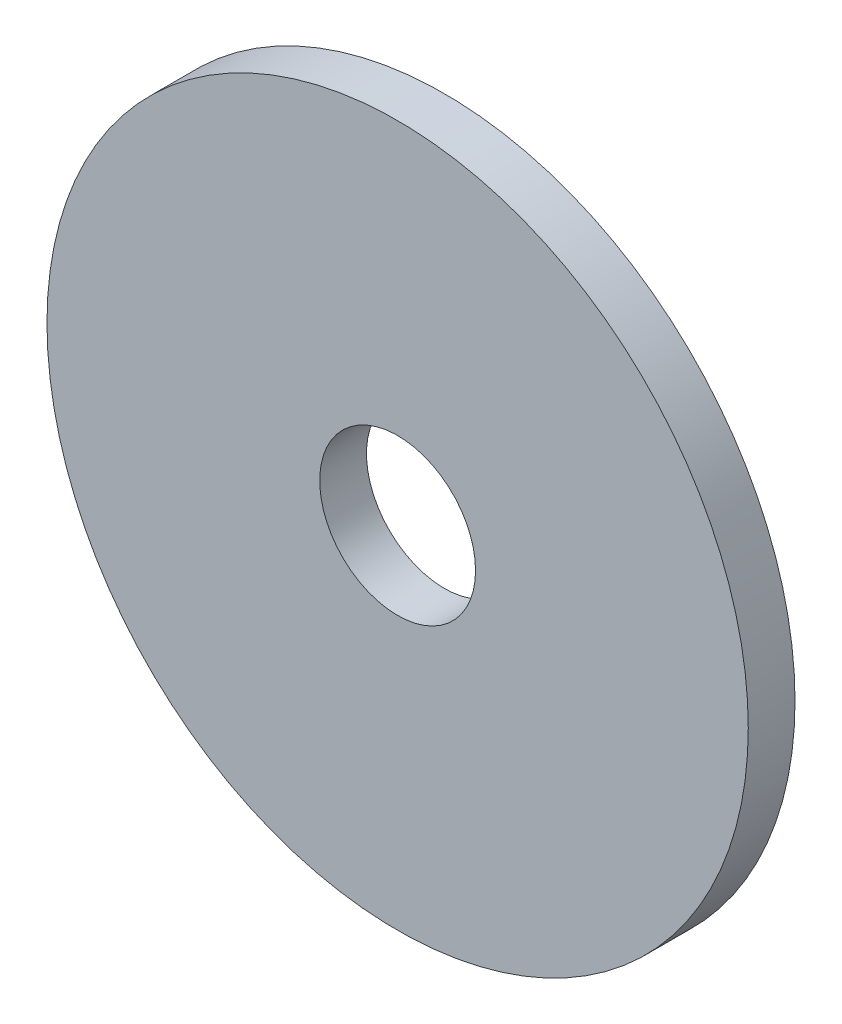
SolidWorks part; units mm, degrees
ref_plane "前视基准面" through (0, 0, 0) normal (0, 0, 1) x (1, 0, 0)
ref_plane "上视基准面" through (0, 0, 0) normal (0, 1, 0) x (1, 0, 0)
ref_plane "右视基准面" through (0, 0, 0) normal (1, 0, 0) x (0, 0, -1)
sketch "草图1" plane through (0, 0, 0) normal (0, 0, 1) x (1, 0, 0)
  circle A0 centre (0, 0) radius 22.5
  circle A1 centre (0, 0) radius 5
extrude "凸台-拉伸1" add sketch "草图1" along normal blind 3
